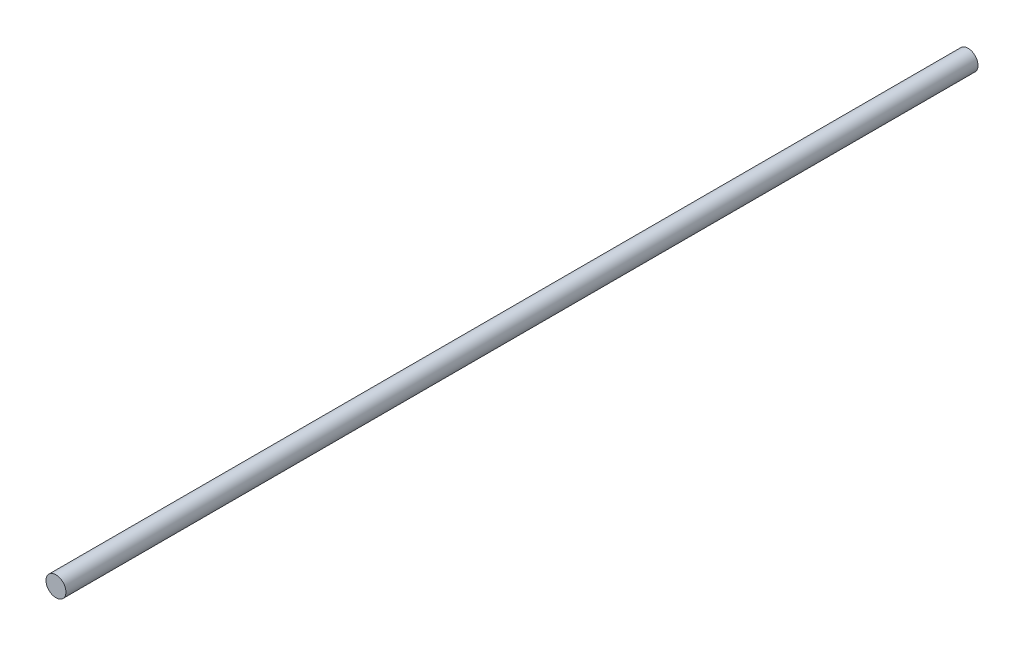
from build123d import *

# Parameters (mm, degrees)
SKETCH1_R           = 1.44
BOSS_EXTRUDE1_DEPTH = 131.6


with BuildPart() as part:
    # Sketch1 → Boss-Extrude1 (new body)
    with BuildSketch(Plane.XY):
        Circle(SKETCH1_R)
    extrude(amount=BOSS_EXTRUDE1_DEPTH)


solid = part.part
